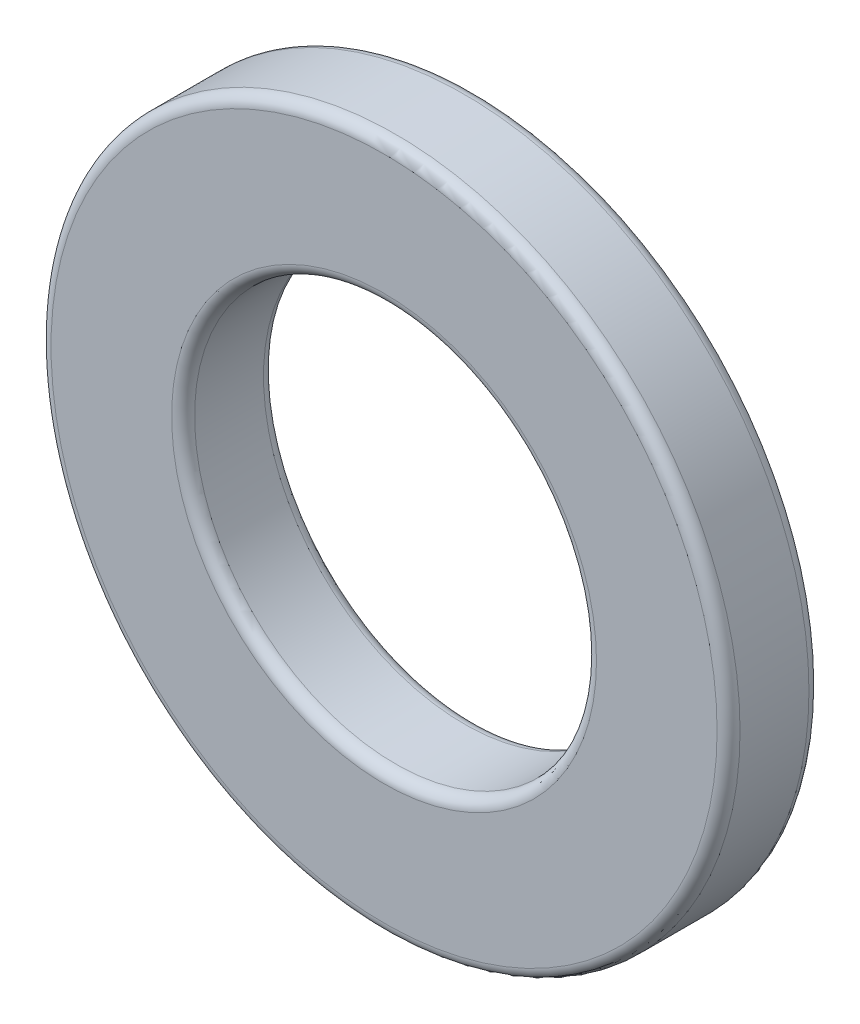
from build123d import *

# Parameters (mm, degrees)
SKETCH_1_R      = 30
SKETCH_1_R_2    = 17.5
EXTRUDE_1_DEPTH = 8
FILLET_1_R      = 1


with BuildPart() as part:
    # 草图1 → 凸台-拉伸1 (new body)
    with BuildSketch(Plane.XY):
        Circle(SKETCH_1_R)
        Circle(SKETCH_1_R_2, mode=Mode.SUBTRACT)
    extrude(amount=EXTRUDE_1_DEPTH)

    # 圆角1
    fillet_1_edges = [part.edges().sort_by_distance(p)[0] for p in [
        (-30, 0, 0),
        (-30, 0, 8),
        (-17.5, 0, 0),
        (-17.5, 0, 8),
    ]]
    fillet(fillet_1_edges, radius=FILLET_1_R)


solid = part.part
